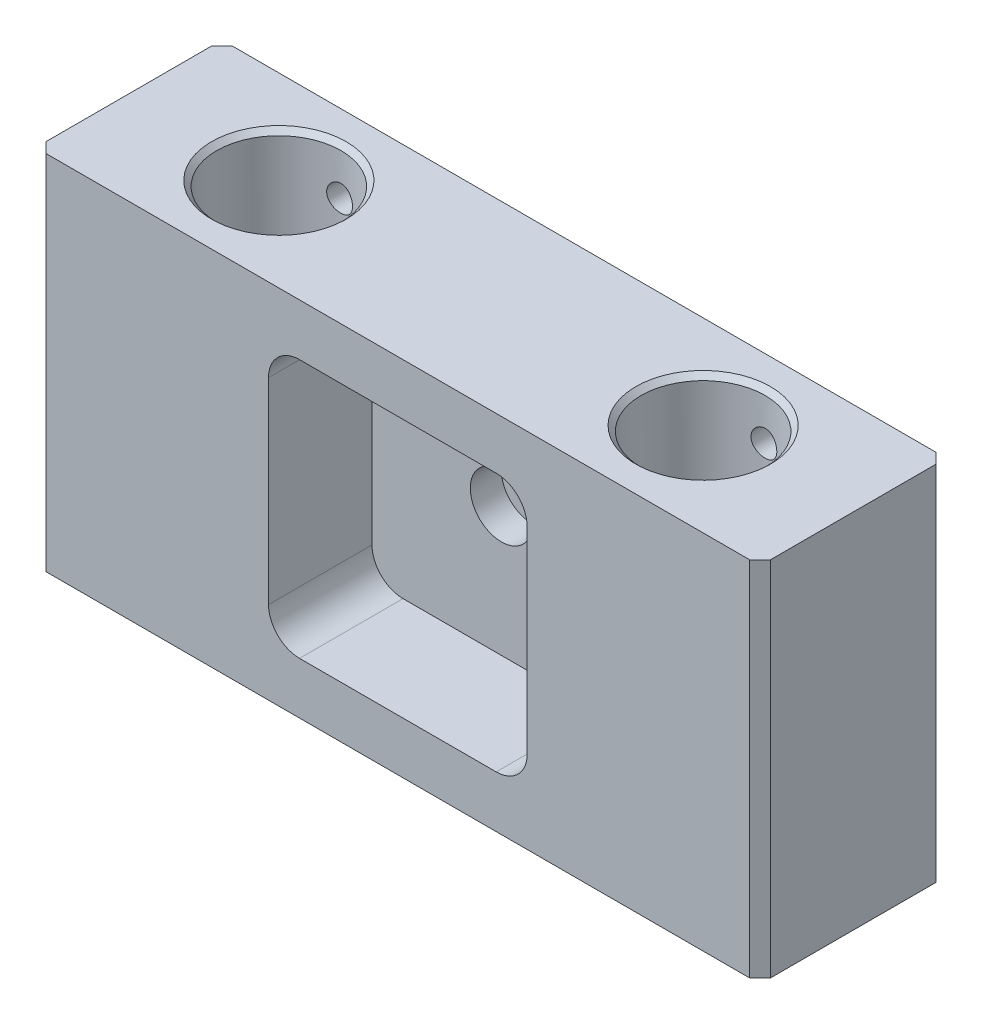
SolidWorks part; units mm, degrees
material "A6063"
ref_plane "Front Plane" through (0, 0, 0) normal (0, 0, 1) x (1, 0, 0)
ref_plane "Top Plane" through (0, 0, 0) normal (0, 1, 0) x (1, 0, 0)
ref_plane "Right Plane" through (0, 0, 0) normal (1, 0, 0) x (0, 0, -1)
sketch "Sketch1" plane through (0, 0, 0) normal (0, 0, 1) x (1, 0, 0)
  line L1 (-35, 17.5) -> (35, 17.5)
  line L2 (-35, 17.5) -> (-35, -17.5)
  line L3 (-35, -17.5) -> (35, -17.5)
  line L4 (35, 17.5) -> (35, -17.5)
  line L5 (-35, 17.5) -> (35, -17.5) construction
  line L6 (-35, -17.5) -> (35, 17.5) construction
  point P0 (0, 0)
  dimension "D1" = 70
  dimension "D2" = 35
extrude "Boss-Extrude1" add sketch "Sketch1" along normal mid plane 18
sketch "Sketch2" plane through (0, 0, 9) normal (0, 0, 1) x (1, 0, 0)
  line L1 (-9.5, 12.5) -> (9.5, 12.5)
  line L2 (-12.5, 9.5) -> (-12.5, -9.5)
  line L3 (-9.5, -12.5) -> (9.5, -12.5)
  line L4 (12.5, 9.5) -> (12.5, -9.5)
  line L5 (-12.5, 12.5) -> (12.5, -12.5) construction
  line L6 (-12.5, -12.5) -> (12.5, 12.5) construction
  line L13 (0, 17.5) -> (0, -17.5) construction
  line L14 (35, 17.5) -> (-35, 17.5) construction
  line L15 (-35, -17.5) -> (35, -17.5) construction
  arc A0 (12.5, 9.5) -> (9.5, 12.5) centre (9.5, 9.5) ccw
  arc A1 (12.5, -9.5) -> (9.5, -12.5) centre (9.5, -9.5) cw
  arc A2 (-9.5, -12.5) -> (-12.5, -9.5) centre (-9.5, -9.5) cw
  arc A3 (-9.5, 12.5) -> (-12.5, 9.5) centre (-9.5, 9.5) ccw
  point P0 (0, 0)
  dimension "D3" = 3
  dimension "D1" = 25
  dimension "D2" = 25
extrude "Cut-Extrude1" cut sketch "Sketch2" against normal blind 10
sketch "Sketch3" plane through (0, 17.5, 0) normal (0, 1, 0) x (1, 0, 0)
  line L0 (0, 9) -> (0, -9) construction
  line L1 (35, 9) -> (-35, 9) construction
  line L2 (35, -9) -> (-35, -9) construction
  circle A0 centre (-20.5, 0) radius 6
  circle A1 centre (20.5, 0) radius 6
  dimension "D1" = 41
  dimension "D2" = 12
extrude "Cut-Extrude2" cut sketch "Sketch3" against normal through all
hole_wizard "M3 Tapped Hole1" positions "Sketch5" profile "Sketch4" tap size "M3" standard "GB"
sketch "Sketch5" plane through (0, 0, -9) normal (0, 0, -1) x (-1, 0, 0)
  line L0 (0, 17.5) -> (0, -17.5) construction
  line L1 (-35, 17.5) -> (35, 17.5) construction
  line L2 (35, -17.5) -> (-35, -17.5) construction
  line L4 (-35, 0) -> (35, 0) construction
  line L5 (-35, -17.5) -> (-35, 17.5) construction
  line L6 (35, 17.5) -> (35, -17.5) construction
  point P0 (-20.5, 13)
  point P1 (-20.5, -13)
  point P3 (20.5, -13)
  point P5 (20.5, 13)
  dimension "D1" = 26
  dimension "D2" = 41
sketch "Sketch4" plane through (20.5, 13, -9) normal (1, 0, 0) x (0, 1, 0)
  line L0 (0, 0) -> (0, 3)
  line L1 (0, 3) -> (1.25, 3)
  line L2 (1.25, 3) -> (1.25, 0)
  line L5 (1.25, 0) -> (0, 0)
  line L11 (0, -6.35) -> (0, 107.95) construction
  dimension "通孔螺纹孔钻头直径" = 2.5
  dimension "通孔螺纹孔钻头深度" = 3
cosmetic thread "Hole thread1" parameters "D2"=3
cosmetic thread "Hole thread2" parameters "D2"=3
cosmetic thread "Hole thread3" parameters "D2"=3
cosmetic thread "Hole thread4" parameters "D2"=3
hole_wizard "CBORE for M3 Hex Head Bolt1" positions "Sketch8" profile "Sketch7" counterbore size "M3" standard "GB" end condition through all
sketch "Sketch8" plane through (-21.2233, -7.5873, -1) normal (0, 0, 1) x (1, 0, 0)
  line L0 (-13.7767, 25.0873) -> (-13.7767, -9.9127) construction
  point P4 (21.2233, 7.5873)
  point P13 (-13.7767, 7.5873)
  dimension "D2" = 35
sketch "Sketch7" plane through (0, 0, -1) normal (1, 0, 0) x (0, -1, 0)
  line L0 (0, 0) -> (0, 8)
  line L1 (0, 8) -> (1.75, 8)
  line L3 (1.75, 8) -> (1.75, 3)
  line L4 (1.75, 3) -> (3, 3)
  line L5 (3, 3) -> (3, 0)
  line L7 (3, 0) -> (0, 0)
  line L11 (0, -6.35) -> (0, 107.95) construction
  dimension "通孔孔直径" = 3.5
  dimension "通孔孔深度" = 8
  dimension "柱形沉头孔直径" = 6
  dimension "柱形沉头孔深度" = 3
sketch "Sketch9" plane through (0, 0, -9) normal (0, 0, -1) x (-1, 0, 0)
  circle A1 centre (0, 0) radius 3
  dimension "D1" = 6
extrude "Cut-Extrude3" cut sketch "Sketch9" against normal blind 3
chamfer "Chamfer1" distance 1 angle 45 4 edges at (-35, 0, -9) (-35, 0, 9) (35, 0, -9) (35, 0, 9)
chamfer "Chamfer2" distance 0.5 angle 45 4 edges at (-20.5, -17.5, 6) (20.5, -17.5, 6) (20.5, 17.5, 6) (-20.5, 17.5, 6)
